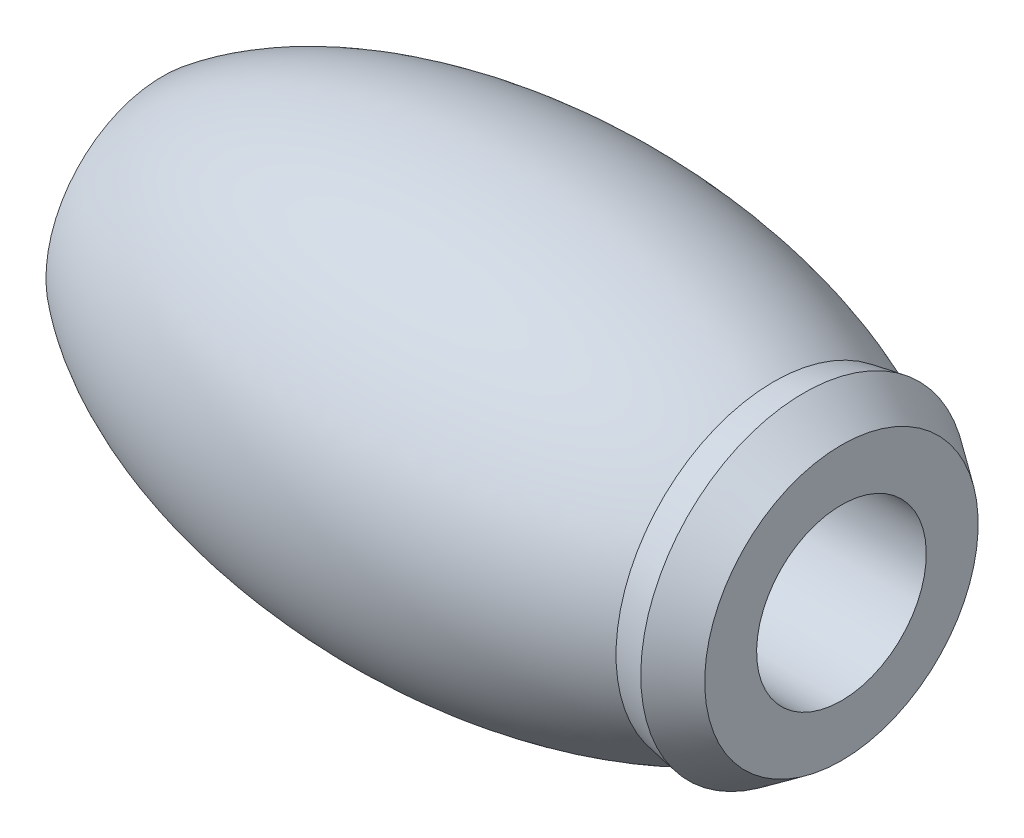
from build123d import *

# Parameters (mm, degrees)
SKETCH2_R           = 20
SKETCH2_R_2         = 13.75831161
BOSS_EXTRUDE2_DEPTH = 9.864364
BOSS_EXTRUDE2_DRAFT = -10
CHAMFER2_SIZE       = 4.5
CHAMFER2_SIZE2      = 3.884480955


with BuildPart() as part:
    # Sketch1 → Revolve2 (revolve)
    with BuildSketch(Plane.XY, mode=Mode.PRIVATE) as revolve2_sk:
        with BuildLine():
            Line((-40, 10), (40, 10))
            add(Edge.make_bspline(
                [(40, 10), (0, 48.4), (-40, 10)],
                knots=[0.471861837, 0.471861837, 0.471861837, 2.669730816, 2.669730816, 2.669730816], degree=2, weights=[1, 0.454545455, 1]))
        make_face()
        with BuildLine():
            Line((-40, 13.75831161), (-40, 10))
            add(Edge.make_bspline(
                [(40, 10), (0, 48.4), (-40, 10)],
                knots=[0.471861837, 0.471861837, 0.471861837, 2.669730816, 2.669730816, 2.669730816], degree=2, weights=[1, 0.454545455, 1]))
            Line((40, 10), (40, 13.75831161))
            add(Edge.make_bspline(
                [(40, 13.75831161), (25.800917492, 25), (0, 25)],
                knots=[0.582762373, 0.582762373, 0.582762373, 1.570796327, 1.570796327, 1.570796327], degree=2, weights=[1, 0.775166232, 0.775166232]))
            add(Edge.make_bspline(
                [(0, 25), (-25.800917492, 25), (-40, 13.75831161)],
                knots=[1.570796327, 1.570796327, 1.570796327, 2.558830281, 2.558830281, 2.558830281], degree=2, weights=[0.775166232, 0.775166232, 1]))
        make_face()
    revolve(revolve2_sk.sketch.rotate(Axis((42.752815742, 0, 0), (1, 0, 0)), 180), axis=Axis((42.752815742, 0, 0), (1, 0, 0)))


with BuildPart() as boss_extrude2_tool:
    # Sketch2 → Boss-Extrude2 (with draft: the straight prism first)
    with BuildSketch(Plane(origin=(40, 0, 0), x_dir=(0, 0, -1), z_dir=(1, 0, 0))):
        Circle(SKETCH2_R)
        Circle(SKETCH2_R_2, mode=Mode.SUBTRACT)
    extrude(amount=-BOSS_EXTRUDE2_DEPTH)
    # Boss-Extrude2: the draft: its side faces are tilted about the plane it starts from
    boss_extrude2_sides = [boss_extrude2_tool.faces().sort_by_distance(p)[0] for p in [
        (35.067818, 0, 20),
        (35.067818, 0, 13.75831161),
    ]]
    draft(boss_extrude2_sides, Plane(origin=(40, 0, 0), x_dir=(0, 0, -1), z_dir=(1, 0, 0)), BOSS_EXTRUDE2_DRAFT)


with BuildPart() as part_1:
    add(part.part)

    # Boss-Extrude2: add boss_extrude2_tool
    add(boss_extrude2_tool.part)

    # Chamfer2
    chamfer2_edges = [part_1.edges().sort_by_distance(p)[0] for p in [
        (40, 0, 20),
    ]]
    chamfer2_side = [part_1.faces().sort_by_distance(p)[0] for p in [
        (36.012111156, 0, 19.296827601),
    ]]
    chamfer(chamfer2_edges, length=CHAMFER2_SIZE, length2=CHAMFER2_SIZE2, reference=chamfer2_side[0])


solid = part_1.part
